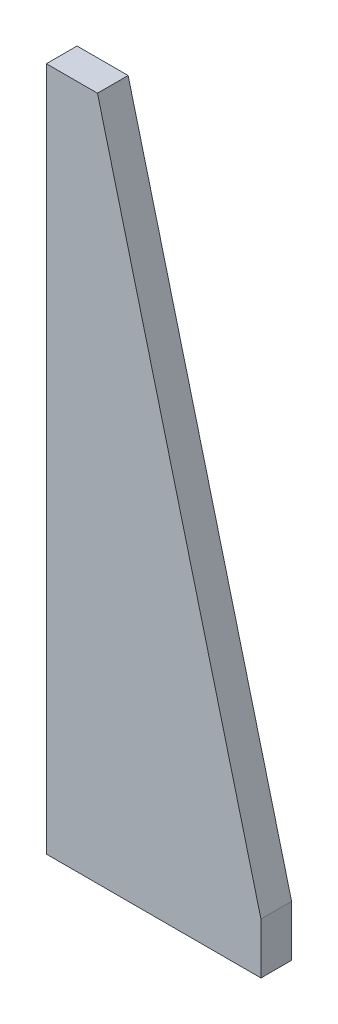
from build123d import *

# Parameters (mm, degrees)
EXTRUDE_1_DEPTH = 30


with BuildPart() as part:
    # 草图1 → 凸台-拉伸1 (new body)
    with BuildSketch(Plane.XY):
        Polygon((0, 0), (0, 670), (50, 670), (210, 50), (210, 0), align=None)
    extrude(amount=EXTRUDE_1_DEPTH)


solid = part.part
